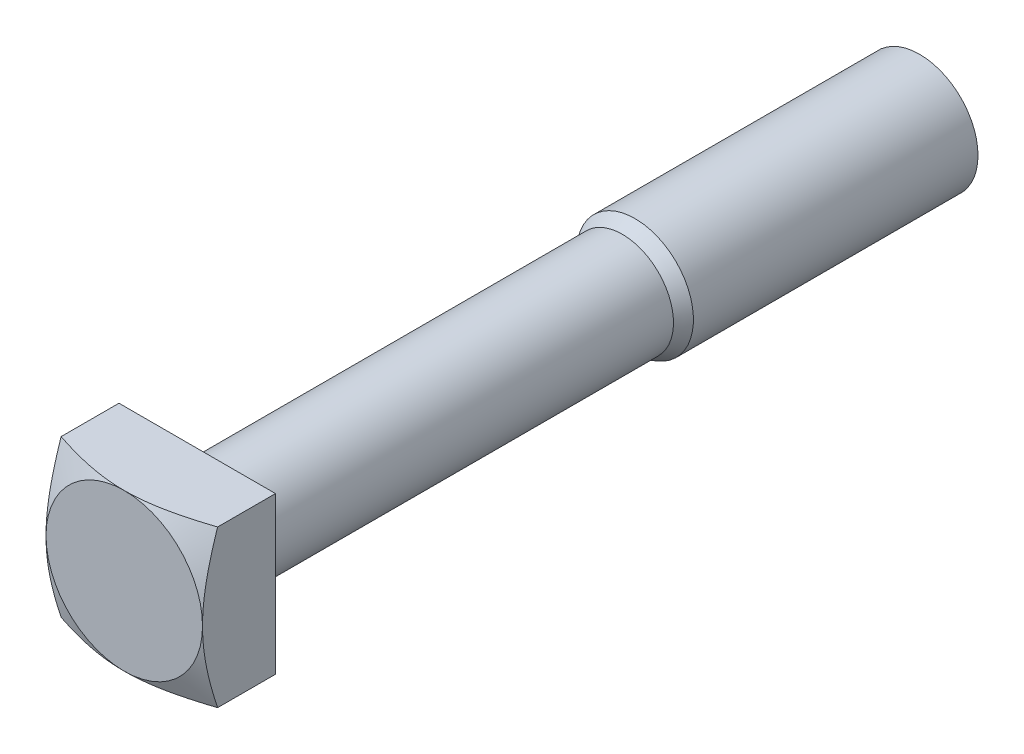
from build123d import *

# Parameters (mm, degrees)
SKETCH1_W          = 32.173358544
SKETCH1_H          = 32.173358544
BASE_EXTRUDE_DEPTH = 15
SKETCH4_OUTSIDE_W  = 164.92
SKETCH4_OUTSIDE_H  = 164.92
SKETCH4_OUTSIDE_R  = 16.086679272
CUT_EXTRUDE1_DEPTH = 28.25
CUT_EXTRUDE1_DRAFT = -65
FILLET1_R          = 0.8


with BuildPart() as part:
    # Sketch1 → Base-Extrude (new body)
    with BuildSketch(Plane.XY):
        Rectangle(SKETCH1_W, SKETCH1_H)
    extrude(amount=BASE_EXTRUDE_DEPTH)


with BuildPart() as cut_extrude1_tool:
    # Sketch4 outside → Cut-Extrude1 (with draft: the straight prism first)
    with BuildSketch(Plane.XY.offset(15)):
        Rectangle(SKETCH4_OUTSIDE_W, SKETCH4_OUTSIDE_H)
        Circle(SKETCH4_OUTSIDE_R, mode=Mode.SUBTRACT)
    extrude(amount=-CUT_EXTRUDE1_DEPTH)
    # Cut-Extrude1: the draft: its side faces are tilted about the plane it starts from
    cut_extrude1_sides = [cut_extrude1_tool.faces().sort_by_distance(p)[0] for p in [
        (0, -82.46, 0.875),
        (82.46, 0, 0.875),
        (0, 82.46, 0.875),
        (-82.46, 0, 0.875),
        (-16.086679272, 0, 0.875),
    ]]
    draft(cut_extrude1_sides, Plane.XY.offset(15), CUT_EXTRUDE1_DRAFT)


with BuildPart() as part_1:
    add(part.part)

    # Cut-Extrude1: cut by cut_extrude1_tool
    add(cut_extrude1_tool.part, mode=Mode.SUBTRACT)

    # Sketch2 → Boss-Revolve1 (revolve)
    with BuildSketch(Plane(origin=(0, 0, 0), x_dir=(1, 0, 0), z_dir=(0, 1, 0)), mode=Mode.PRIVATE) as boss_revolve1_sk:
        Polygon((0, 0), (10.5, 0), (10.5, 87.401923789), (12, 90), (12, 150), (0, 150), align=None)
    revolve(boss_revolve1_sk.sketch.rotate(Axis((0, 0, -150), (0, 0, 1)), 180), axis=Axis((0, 0, -150), (0, 0, 1)))

    # Fillet1
    fillet1_edges = [part_1.edges().sort_by_distance(p)[0] for p in [
        (10.5, 0, 0),
    ]]
    fillet(fillet1_edges, radius=FILLET1_R)

    # Sketch3 → Cut-Revolve1 (revolve, cut)
    with BuildSketch(Plane(origin=(0, 0, 0), x_dir=(1, 0, 0), z_dir=(0, 1, 0))):
        Polygon((9.402, 150), (12, 151.499955999), (12, 148.500044001), align=None)
    revolve(axis=Axis((0, 0, 0), (0, 0, -1)), mode=Mode.SUBTRACT)


solid = part_1.part
